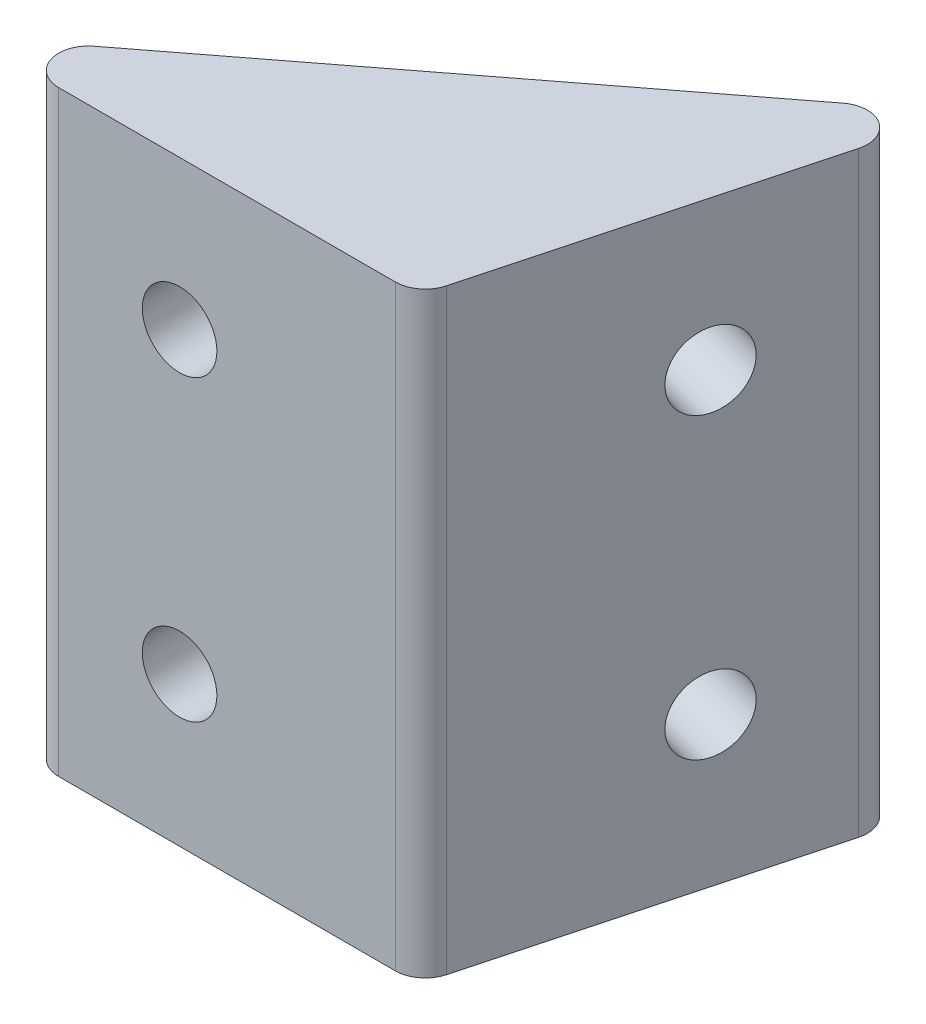
from build123d import *

# Parameters (mm, degrees)
EXTRUDE_1_DEPTH             = 20
HOLE_WIZARD_M3_1_AT_2_COUNT = 2
HOLE_WIZARD_M3_1_AT_2_PITCH = 10
FILLET_1_R                  = 1


with BuildPart() as part:
    # 草图1 → 凸台-拉伸1 (new body)
    with BuildSketch(Plane(origin=(0, 0, 0), x_dir=(1, 0, 0), z_dir=(0, 1, 0))):
        Polygon((0, 0), (15, 0), (18.882285677, 14.488887394), align=None)
    extrude(amount=EXTRUDE_1_DEPTH)

    # 草图4 → M3 螺纹孔1 (revolve, cut)
    with BuildSketch(Plane(origin=(17.070552361, 15, -7.72740661), x_dir=(0.25881904510251796, 0, -0.9659258262890691), z_dir=(0, 1, 0))):
        Polygon((0, 0), (0, 7.5), (1.25, 6.748924226), (1.25, 0), align=None)
    hole_wizard_m3_1 = revolve(axis=Axis((23.204181358, 15, -6.083905674), (-0.9659258262890691, 0, -0.2588190451025179)), mode=Mode.SUBTRACT)

    # M3 螺纹孔1 at 2: M3 螺纹孔1 ×2
    with Locations(*[(0, -i * HOLE_WIZARD_M3_1_AT_2_PITCH, 0) for i in range(1, HOLE_WIZARD_M3_1_AT_2_COUNT)]):
        add(hole_wizard_m3_1, mode=Mode.SUBTRACT)

    # 镜向1: M3 螺纹孔1 across plane
    add(hole_wizard_m3_1.mirror(Plane(origin=(9.441142838, 0, -7.244443697), x_dir=(0.6087614290087218, 0, 0.7933533402912344), z_dir=(0.7933533402912343, 0, -0.6087614290087218))), mode=Mode.SUBTRACT)

    # 镜向1 copy 1 sketch → 镜向1 copy 1 (revolve, cut)
    with BuildSketch(Plane(origin=(7, 5, 0), x_dir=(-1, 0, 0), z_dir=(0, 1, 0))):
        Polygon((0, 0), (0, -7.5), (1.25, -6.748924226), (1.25, 0), align=None)
    revolve(axis=Axis((7, 5, 6.35), (0, 0, 1)), mode=Mode.SUBTRACT)

    # 圆角1
    fillet_1_edges = [part.edges().sort_by_distance(p)[0] for p in [
        (18.882285677, 10, -14.488887394),
        (15, 10, 0),
        (0, 10, 0),
    ]]
    fillet(fillet_1_edges, radius=FILLET_1_R)


solid = part.part
